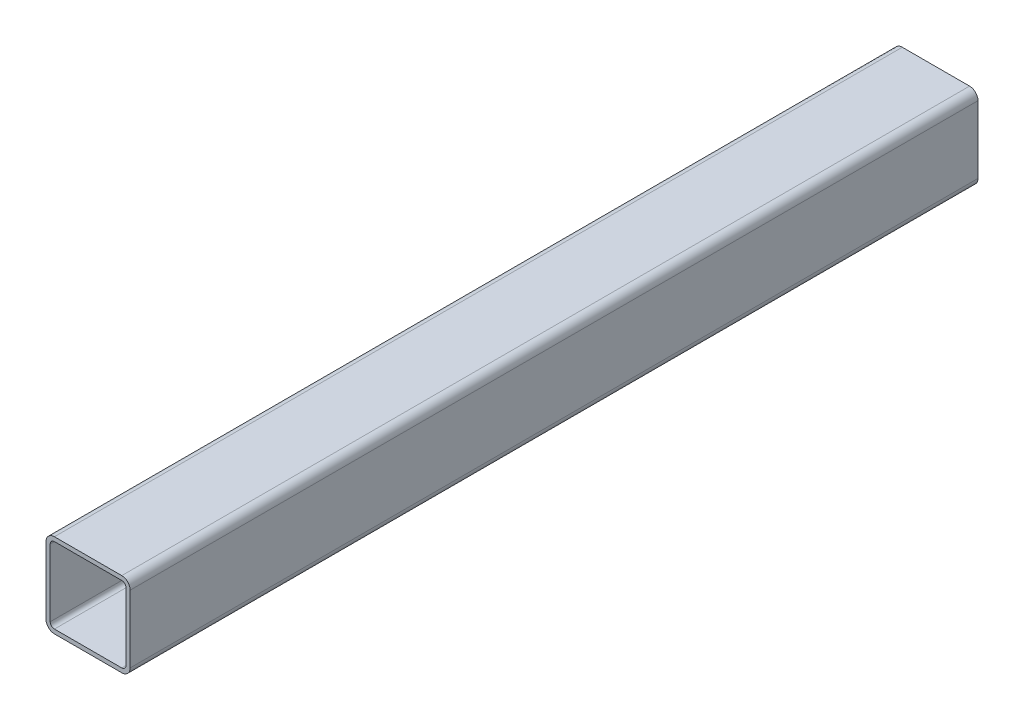
SolidWorks part; units mm, degrees
material "Q235A"
ref_plane "Front Plane" through (0, 0, 0) normal (0, 0, 1) x (1, 0, 0)
ref_plane "Top Plane" through (0, 0, 0) normal (0, 1, 0) x (1, 0, 0)
ref_plane "Right Plane" through (0, 0, 0) normal (1, 0, 0) x (0, 0, -1)
sketch "Sketch1" plane through (0, 0, 0) normal (0, 0, 1) x (1, 0, 0)
  line L1 (-20, 20) -> (20, 20)
  line L2 (-20, 20) -> (-20, -20)
  line L3 (-20, -20) -> (20, -20)
  line L4 (20, 20) -> (20, -20)
  line L5 (-20, 20) -> (20, -20) construction
  line L6 (-20, -20) -> (20, 20) construction
  line L7 (-18, 18) -> (18, 18)
  line L8 (-18, 18) -> (-18, -18)
  line L9 (-18, -18) -> (18, -18)
  line L10 (18, 18) -> (18, -18)
  line L11 (-18, 18) -> (18, -18) construction
  line L12 (-18, -18) -> (18, 18) construction
  point P0 (0, 0)
  point P6 (0, 0)
  dimension "D1" = 40
  dimension "D2" = 40
  dimension "D3" = 2
  dimension "D4" = 2
extrude "Boss-Extrude1" add sketch "Sketch1" along normal blind 403
fillet "Fillet1" radius 2 4 edges at (18, 18, 201.5) (-18, 18, 201.5) (-18, -18, 201.5) (18, -18, 201.5)
fillet "Fillet2" radius 4 4 edges at (20, 20, 201.5) (20, -20, 201.5) (-20, 20, 201.5) (-20, -20, 201.5)
